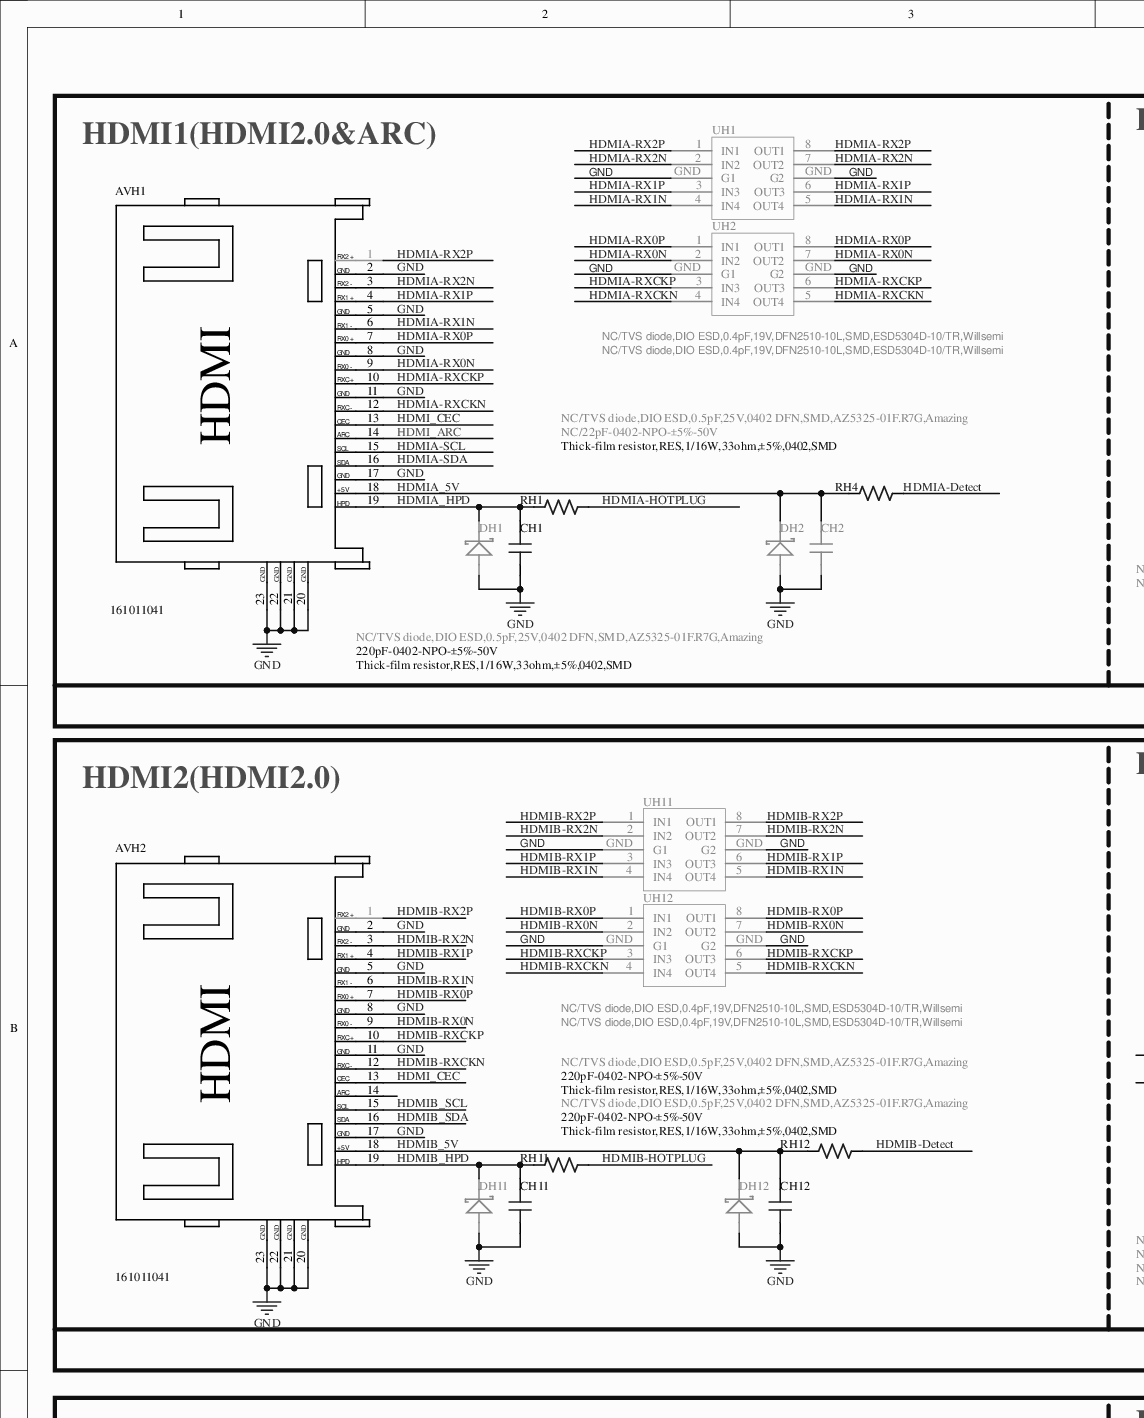
[diagram p0: MISC86290-15.SchDoc, top left]
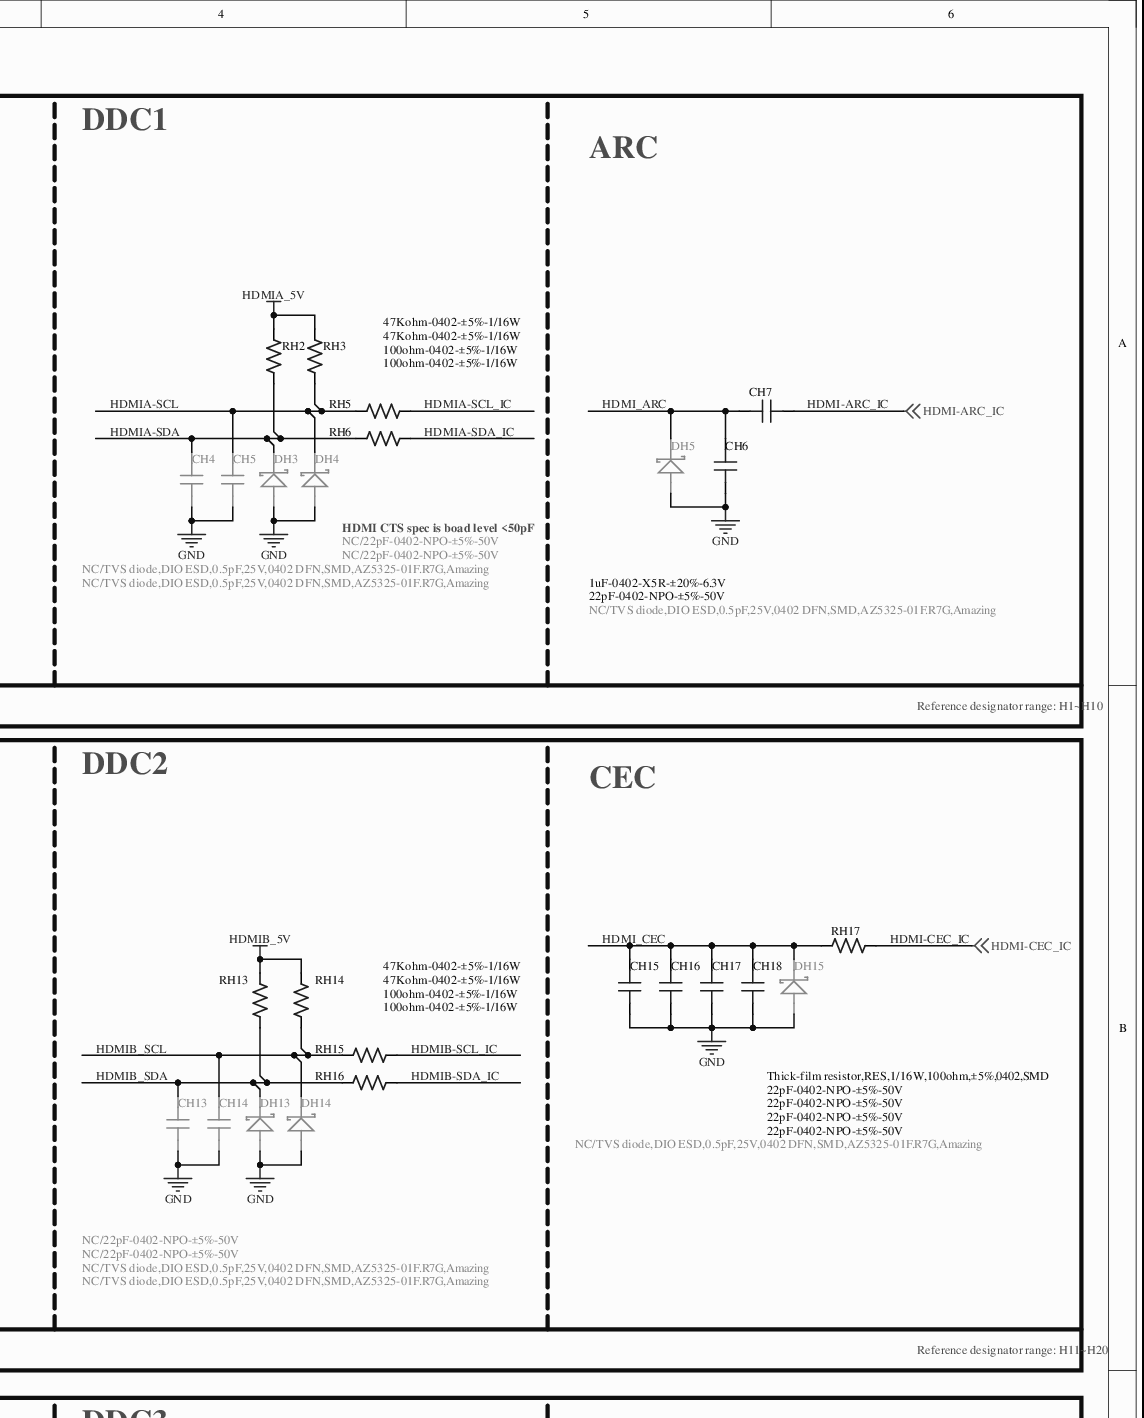
[diagram p1: MISC86290-15.SchDoc, top right]
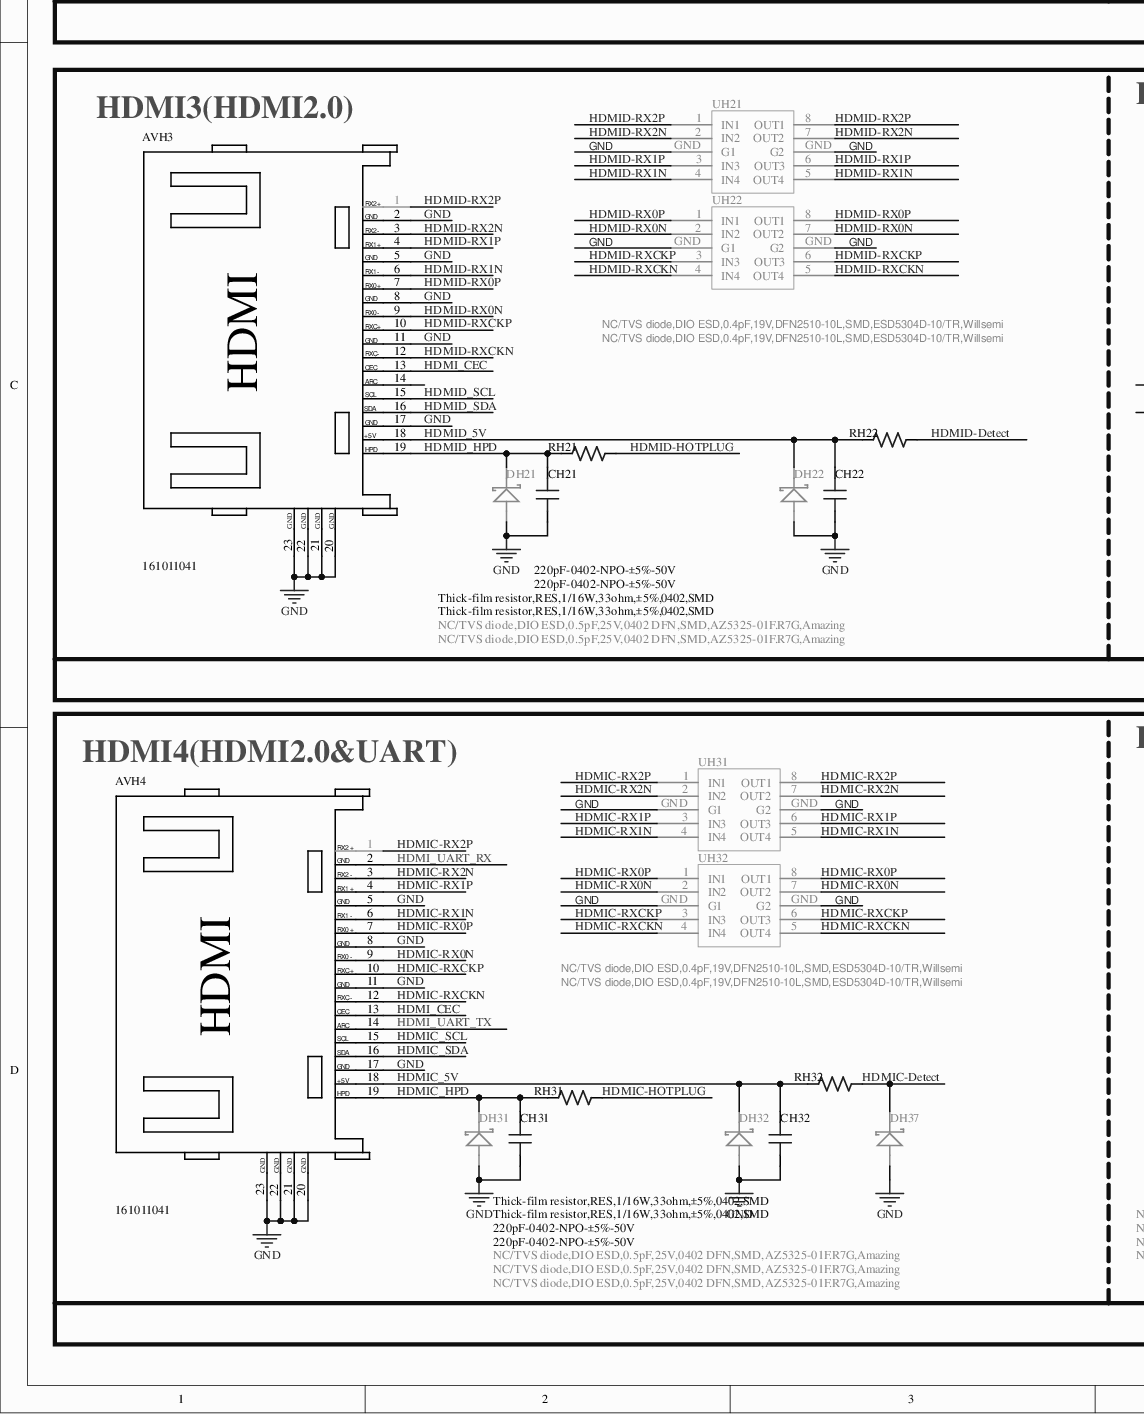
[diagram p2: MISC86290-15.SchDoc, bottom left]
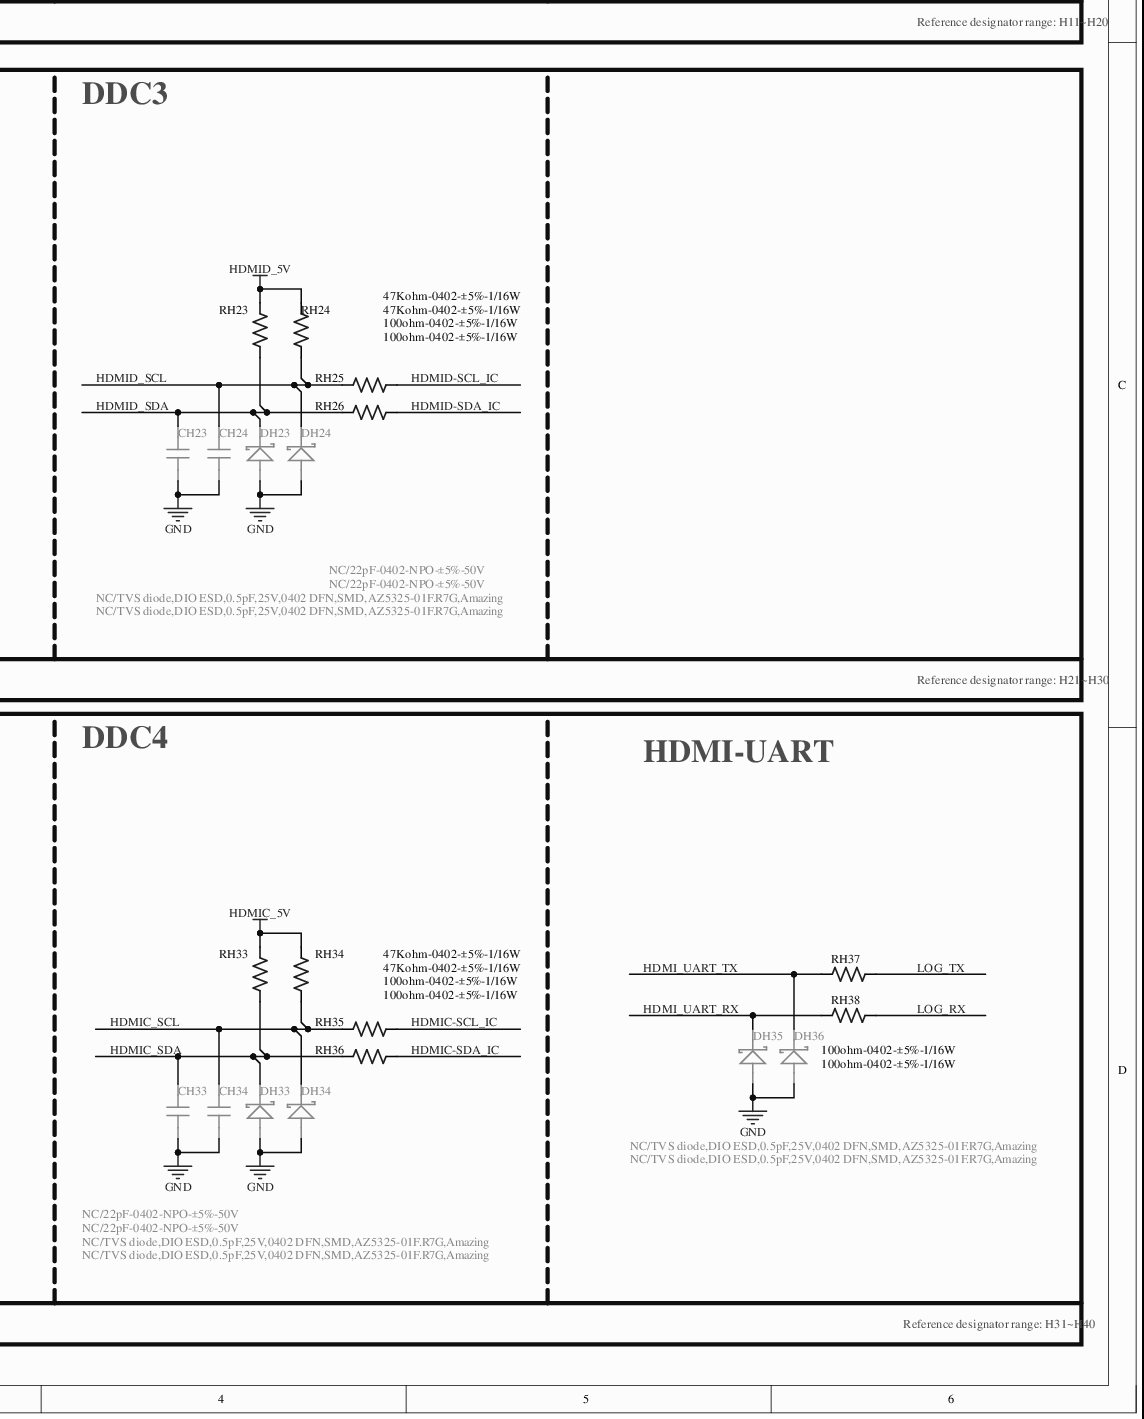
[diagram p3: MISC86290-15.SchDoc, bottom right]
# Altium project MISC86290.PrjPcb (part 11 of 13)

## Sheet MISC86290-15.SchDoc
size 406 x 508 mm

### Parts
AVH1  161011041  [HDMI-HS-1]
AVH2  161011041  [HDMI-HS-1]
AVH3  161011041  [HDMI-HS-1]
AVH4  161011041  [HDMI-HS-1]
CH1  220pF-0402-NPO-±5%-50V  [C0402]
CH2  NC/22pF-0402-NPO-±5%-50V  [C0402]
CH4  NC/22pF-0402-NPO-±5%-50V  [C0402]
CH5  NC/22pF-0402-NPO-±5%-50V  [C0402]
CH6  22pF-0402-NPO-±5%-50V  [C0402]
CH7  1uF-0402-X5R-±20%-6.3V  [C0402]
CH11  220pF-0402-NPO-±5%-50V  [C0402]
CH12  220pF-0402-NPO-±5%-50V  [C0402]
CH13  NC/22pF-0402-NPO-±5%-50V  [C0402]
CH14  NC/22pF-0402-NPO-±5%-50V  [C0402]
CH15  22pF-0402-NPO-±5%-50V  [C0402]
CH16  22pF-0402-NPO-±5%-50V  [C0402]
CH17  22pF-0402-NPO-±5%-50V  [C0402]
CH18  22pF-0402-NPO-±5%-50V  [C0402]
CH21  220pF-0402-NPO-±5%-50V  [C0402]
CH22  220pF-0402-NPO-±5%-50V  [C0402]
CH23  NC/22pF-0402-NPO-±5%-50V  [C0402]
CH24  NC/22pF-0402-NPO-±5%-50V  [C0402]
CH31  220pF-0402-NPO-±5%-50V  [C0402]
CH32  220pF-0402-NPO-±5%-50V  [C0402]
CH33  NC/22pF-0402-NPO-±5%-50V  [C0402]
CH34  NC/22pF-0402-NPO-±5%-50V  [C0402]
DH1  NC/TVS diode,DIO ESD,0.5pF,25V,0402 DFN,SMD,AZ5325-01F.R7G,Amazing  [DIODE-S0402]
DH2  NC/TVS diode,DIO ESD,0.5pF,25V,0402 DFN,SMD,AZ5325-01F.R7G,Amazing  [DIODE-S0402]
DH3  NC/TVS diode,DIO ESD,0.5pF,25V,0402 DFN,SMD,AZ5325-01F.R7G,Amazing  [DIODE-S0402]
DH4  NC/TVS diode,DIO ESD,0.5pF,25V,0402 DFN,SMD,AZ5325-01F.R7G,Amazing  [DIODE-S0402]
DH5  NC/TVS diode,DIO ESD,0.5pF,25V,0402 DFN,SMD,AZ5325-01F.R7G,Amazing  [DIODE-S0402]
DH11  NC/TVS diode,DIO ESD,0.5pF,25V,0402 DFN,SMD,AZ5325-01F.R7G,Amazing  [DIODE-S0402]
DH12  NC/TVS diode,DIO ESD,0.5pF,25V,0402 DFN,SMD,AZ5325-01F.R7G,Amazing  [DIODE-S0402]
DH13  NC/TVS diode,DIO ESD,0.5pF,25V,0402 DFN,SMD,AZ5325-01F.R7G,Amazing  [DIODE-S0402]
DH14  NC/TVS diode,DIO ESD,0.5pF,25V,0402 DFN,SMD,AZ5325-01F.R7G,Amazing  [DIODE-S0402]
DH15  NC/TVS diode,DIO ESD,0.5pF,25V,0402 DFN,SMD,AZ5325-01F.R7G,Amazing  [DIODE-S0402]
DH21  NC/TVS diode,DIO ESD,0.5pF,25V,0402 DFN,SMD,AZ5325-01F.R7G,Amazing  [DIODE-S0402]
DH22  NC/TVS diode,DIO ESD,0.5pF,25V,0402 DFN,SMD,AZ5325-01F.R7G,Amazing  [DIODE-S0402]
DH23  NC/TVS diode,DIO ESD,0.5pF,25V,0402 DFN,SMD,AZ5325-01F.R7G,Amazing  [DIODE-S0402]
DH24  NC/TVS diode,DIO ESD,0.5pF,25V,0402 DFN,SMD,AZ5325-01F.R7G,Amazing  [DIODE-S0402]
DH31  NC/TVS diode,DIO ESD,0.5pF,25V,0402 DFN,SMD,AZ5325-01F.R7G,Amazing  [DIODE-S0402]
DH32  NC/TVS diode,DIO ESD,0.5pF,25V,0402 DFN,SMD,AZ5325-01F.R7G,Amazing  [DIODE-S0402]
DH33  NC/TVS diode,DIO ESD,0.5pF,25V,0402 DFN,SMD,AZ5325-01F.R7G,Amazing  [DIODE-S0402]
DH34  NC/TVS diode,DIO ESD,0.5pF,25V,0402 DFN,SMD,AZ5325-01F.R7G,Amazing  [DIODE-S0402]
DH35  NC/TVS diode,DIO ESD,0.5pF,25V,0402 DFN,SMD,AZ5325-01F.R7G,Amazing  [DIODE-S0402]
DH36  NC/TVS diode,DIO ESD,0.5pF,25V,0402 DFN,SMD,AZ5325-01F.R7G,Amazing  [DIODE-S0402]
DH37  NC/TVS diode,DIO ESD,0.5pF,25V,0402 DFN,SMD,AZ5325-01F.R7G,Amazing  [DIODE-S0402]
RH1  Thick-film resistor,RES,1/16W,33ohm,±5%,0402,SMD  [R0402]
RH2  47Kohm-0402-±5%-1/16W  [R0402]
RH3  47Kohm-0402-±5%-1/16W  [R0402]
RH4  Thick-film resistor,RES,1/16W,33ohm,±5%,0402,SMD  [R0402]
RH5  100ohm-0402-±5%-1/16W  [R0402]
RH6  100ohm-0402-±5%-1/16W  [R0402]
RH11  Thick-film resistor,RES,1/16W,33ohm,±5%,0402,SMD  [R0402]
RH12  Thick-film resistor,RES,1/16W,33ohm,±5%,0402,SMD  [R0402]
RH13  47Kohm-0402-±5%-1/16W  [R0402]
RH14  47Kohm-0402-±5%-1/16W  [R0402]
RH15  100ohm-0402-±5%-1/16W  [R0402]
RH16  100ohm-0402-±5%-1/16W  [R0402]
RH17  Thick-film resistor,RES,1/16W,100ohm,±5%,0402,SMD  [R0402]
RH21  Thick-film resistor,RES,1/16W,33ohm,±5%,0402,SMD  [R0402]
RH22  Thick-film resistor,RES,1/16W,33ohm,±5%,0402,SMD  [R0402]
RH23  47Kohm-0402-±5%-1/16W  [R0402]
RH24  47Kohm-0402-±5%-1/16W  [R0402]
RH25  100ohm-0402-±5%-1/16W  [R0402]
RH26  100ohm-0402-±5%-1/16W  [R0402]
RH31  Thick-film resistor,RES,1/16W,33ohm,±5%,0402,SMD  [R0402]
RH32  Thick-film resistor,RES,1/16W,33ohm,±5%,0402,SMD  [R0402]
RH33  47Kohm-0402-±5%-1/16W  [R0402]
RH34  47Kohm-0402-±5%-1/16W  [R0402]
RH35  100ohm-0402-±5%-1/16W  [R0402]
RH36  100ohm-0402-±5%-1/16W  [R0402]
RH37  100ohm-0402-±5%-1/16W  [R0402]
RH38  100ohm-0402-±5%-1/16W  [R0402]
UH1  NC/TVS diode,DIO ESD,0.4pF,19V,DFN2510-10L,SMD,ESD5304D-10/TR,Willsemi  [RCL0524P]
UH2  NC/TVS diode,DIO ESD,0.4pF,19V,DFN2510-10L,SMD,ESD5304D-10/TR,Willsemi  [RCL0524P]
UH11  NC/TVS diode,DIO ESD,0.4pF,19V,DFN2510-10L,SMD,ESD5304D-10/TR,Willsemi  [RCL0524P]
UH12  NC/TVS diode,DIO ESD,0.4pF,19V,DFN2510-10L,SMD,ESD5304D-10/TR,Willsemi  [RCL0524P]
UH21  NC/TVS diode,DIO ESD,0.4pF,19V,DFN2510-10L,SMD,ESD5304D-10/TR,Willsemi  [RCL0524P]
UH22  NC/TVS diode,DIO ESD,0.4pF,19V,DFN2510-10L,SMD,ESD5304D-10/TR,Willsemi  [RCL0524P]
UH31  NC/TVS diode,DIO ESD,0.4pF,19V,DFN2510-10L,SMD,ESD5304D-10/TR,Willsemi  [RCL0524P]
UH32  NC/TVS diode,DIO ESD,0.4pF,19V,DFN2510-10L,SMD,ESD5304D-10/TR,Willsemi  [RCL0524P]

### Nets
GND: AVH1.2 AVH1.5 AVH1.8 AVH1.11 AVH1.17 AVH1.20 AVH1.21 AVH1.22 AVH1.23 AVH2.2 AVH2.5 AVH2.8 AVH2.11 AVH2.17 AVH2.20 AVH2.21 AVH2.22 AVH2.23 AVH3.2 AVH3.5 AVH3.8 AVH3.11 AVH3.17 AVH3.20 AVH3.21 AVH3.22 AVH3.23 AVH4.5 AVH4.8 AVH4.11 AVH4.17 AVH4.20 AVH4.21 AVH4.22 AVH4.23 CH1.2 CH2.2 CH4.2 CH5.2 CH6.2 CH11.2 CH12.2 CH13.2 CH14.2 CH15.1 CH16.1 CH17.1 CH18.1 CH21.2 CH22.2 CH23.2 CH24.2 CH31.2 CH32.2 CH33.2 CH34.2 DH1.A DH2.A DH3.A DH4.A DH5.A DH11.A DH12.A DH13.A DH14.A DH15.A DH21.A DH22.A DH23.A DH24.A DH31.A DH32.A DH33.A DH34.A DH35.A DH36.A DH37.A UH1.GND(G1) UH2.GND(G1) UH11.GND(G1) UH12.GND(G1) UH21.GND(G1) UH22.GND(G1) UH31.GND(G1) UH32.GND(G1)
HDMIA_5V: AVH1.18 CH2.1 DH2.K RH2.2 RH3.2 RH4.2
HDMIB_5V: AVH2.18 CH12.1 DH12.K RH12.2 RH13.2 RH14.2
HDMIC_5V: AVH4.18 CH32.1 DH32.K RH32.2 RH33.2 RH34.2
HDMID_5V: AVH3.18 CH22.1 DH22.K RH22.2 RH23.2 RH24.2
HDMI-ARC_IC: CH7.2 ; off-sheet HDMI-ARC_IC
HDMI-CEC_IC: RH17.2 ; off-sheet HDMI-CEC_IC
HDMI_ARC: AVH1.14 CH6.1 CH7.1 DH5.K
HDMI_CEC: AVH1.13 AVH2.13 AVH3.13 AVH4.13 CH15.2 CH16.2 CH17.2 CH18.2 DH15.K RH17.1
HDMI_UART_RX: AVH4.2 DH35.K RH38.1
HDMI_UART_TX: AVH4.14 DH36.K RH37.1
HDMIA-Detect: RH4.1
HDMIA-HOTPLUG: RH1.1
HDMIA-RX0N: AVH1.9 UH2.2(IN2) UH2.7(OUT2)
HDMIA-RX0P: AVH1.7 UH2.1(IN1) UH2.8(OUT1)
HDMIA-RX1N: AVH1.6 UH1.4(IN4) UH1.5(OUT4)
HDMIA-RX1P: AVH1.4 UH1.3(IN3) UH1.6(OUT3)
HDMIA-RX2N: AVH1.3 UH1.2(IN2) UH1.7(OUT2)
HDMIA-RX2P: AVH1.1 UH1.1(IN1) UH1.8(OUT1)
HDMIA-RXCKN: AVH1.12 UH2.4(IN4) UH2.5(OUT4)
HDMIA-RXCKP: AVH1.10 UH2.3(IN3) UH2.6(OUT3)
HDMIA-SCL: AVH1.15 CH5.1 DH4.K RH3.1 RH5.1
HDMIA-SCL_IC: RH5.2
HDMIA-SDA: AVH1.16 CH4.1 DH3.K RH2.1 RH6.1
HDMIA-SDA_IC: RH6.2
HDMIA_HPD: AVH1.19 CH1.1 DH1.K RH1.2
HDMIB-Detect: RH12.1
HDMIB-HOTPLUG: RH11.1
HDMIB-RX0N: AVH2.9 UH12.2(IN2) UH12.7(OUT2)
HDMIB-RX0P: AVH2.7 UH12.1(IN1) UH12.8(OUT1)
HDMIB-RX1N: AVH2.6 UH11.4(IN4) UH11.5(OUT4)
HDMIB-RX1P: AVH2.4 UH11.3(IN3) UH11.6(OUT3)
HDMIB-RX2N: AVH2.3 UH11.2(IN2) UH11.7(OUT2)
HDMIB-RX2P: AVH2.1 UH11.1(IN1) UH11.8(OUT1)
HDMIB-RXCKN: AVH2.12 UH12.4(IN4) UH12.5(OUT4)
HDMIB-RXCKP: AVH2.10 UH12.3(IN3) UH12.6(OUT3)
HDMIB-SCL_IC: RH15.2
HDMIB-SDA_IC: RH16.2
HDMIB_HPD: AVH2.19 CH11.1 DH11.K RH11.2
HDMIB_SCL: AVH2.15 CH14.1 DH14.K RH14.1 RH15.1
HDMIB_SDA: AVH2.16 CH13.1 DH13.K RH13.1 RH16.1
HDMIC-Detect: DH37.K RH32.1
HDMIC-HOTPLUG: RH31.1
HDMIC-RX0N: AVH4.9 UH32.2(IN2) UH32.7(OUT2)
HDMIC-RX0P: AVH4.7 UH32.1(IN1) UH32.8(OUT1)
HDMIC-RX1N: AVH4.6 UH31.4(IN4) UH31.5(OUT4)
HDMIC-RX1P: AVH4.4 UH31.3(IN3) UH31.6(OUT3)
HDMIC-RX2N: AVH4.3 UH31.2(IN2) UH31.7(OUT2)
HDMIC-RX2P: AVH4.1 UH31.1(IN1) UH31.8(OUT1)
HDMIC-RXCKN: AVH4.12 UH32.4(IN4) UH32.5(OUT4)
HDMIC-RXCKP: AVH4.10 UH32.3(IN3) UH32.6(OUT3)
HDMIC-SCL_IC: RH35.2
HDMIC-SDA_IC: RH36.2
HDMIC_HPD: AVH4.19 CH31.1 DH31.K RH31.2
HDMIC_SCL: AVH4.15 CH34.1 DH34.K RH34.1 RH35.1
HDMIC_SDA: AVH4.16 CH33.1 DH33.K RH33.1 RH36.1
HDMID-Detect: RH22.1
HDMID-HOTPLUG: RH21.1
HDMID-RX0N: AVH3.9 UH22.2(IN2) UH22.7(OUT2)
HDMID-RX0P: AVH3.7 UH22.1(IN1) UH22.8(OUT1)
HDMID-RX1N: AVH3.6 UH21.4(IN4) UH21.5(OUT4)
HDMID-RX1P: AVH3.4 UH21.3(IN3) UH21.6(OUT3)
HDMID-RX2N: AVH3.3 UH21.2(IN2) UH21.7(OUT2)
HDMID-RX2P: AVH3.1 UH21.1(IN1) UH21.8(OUT1)
HDMID-RXCKN: AVH3.12 UH22.4(IN4) UH22.5(OUT4)
HDMID-RXCKP: AVH3.10 UH22.3(IN3) UH22.6(OUT3)
HDMID-SCL_IC: RH25.2
HDMID-SDA_IC: RH26.2
HDMID_HPD: AVH3.19 CH21.1 DH21.K RH21.2
HDMID_SCL: AVH3.15 CH24.1 DH24.K RH24.1 RH25.1
HDMID_SDA: AVH3.16 CH23.1 DH23.K RH23.1 RH26.1
LOG_RX: RH38.2
LOG_TX: RH37.2

Not connected (* = marked no-connect by the designer): AVH2 14*; AVH3 14*

### Notes on the sheet
- HDMI1(HDMI2.0&ARC)
- DDC1
- ARC
- (near DH4) HDMI CTS spec is boad level <50pF
- Reference designator range: H1~H10
- DDC2
- HDMI2(HDMI2.0)
- CEC
- Reference designator range: H11~H20
- HDMI3(HDMI2.0)
- DDC3
- Reference designator range: H21~H30
- DDC4
- HDMI4(HDMI2.0&UART)
- HDMI-UART
- Reference designator range: H31~H40

### Library data of the parts
AVH1-AVH4 = 161011041-D-HDMI: CN-HDMI-horizontal-#-#
CH1 CH2 CH4-CH6 CH11-CH14 CH21-CH24 CH31-CH34 = 5pF-0402-NPO-±5%-50V-D
CH7 = 2.2uF-0402-X5R-±20%-6.3V-D
CH15-CH18 = 22pF-0402-NPO-±5%-50V-D
DH1-DH5 DH11-DH14 DH21-DH24 DH31-DH37 = TVS管,DIO ESD,0.4pF,11V,SOD882,SMD,PESD5V0F1BL,NXP-D
DH15 = AVLC18S02003-D
RH1 RH4 RH11 RH12 RH21 RH22 RH31 RH32 = 004.002.0000658-D: Thick-film resistor,RES,1/16W,33ohm,±5%,0402,SMD-D
RH2 RH3 RH13 RH14 RH23 RH24 RH33 RH34 = 10Kohm-0402-±5%-1/16W-D
RH5 RH6 RH15 RH16 RH25 RH26 RH35 RH36 = 22ohm-0402-±5%-1/16W-D
RH17 = 200ohm-0402-±5%-1/16W-D
RH37 RH38 = 100ohm-0402-±5%-1/16W-D
UH1 UH2 UH11 UH12 UH21 UH22 UH31 UH32 = ULC0524P-D: RCLAMP0524J